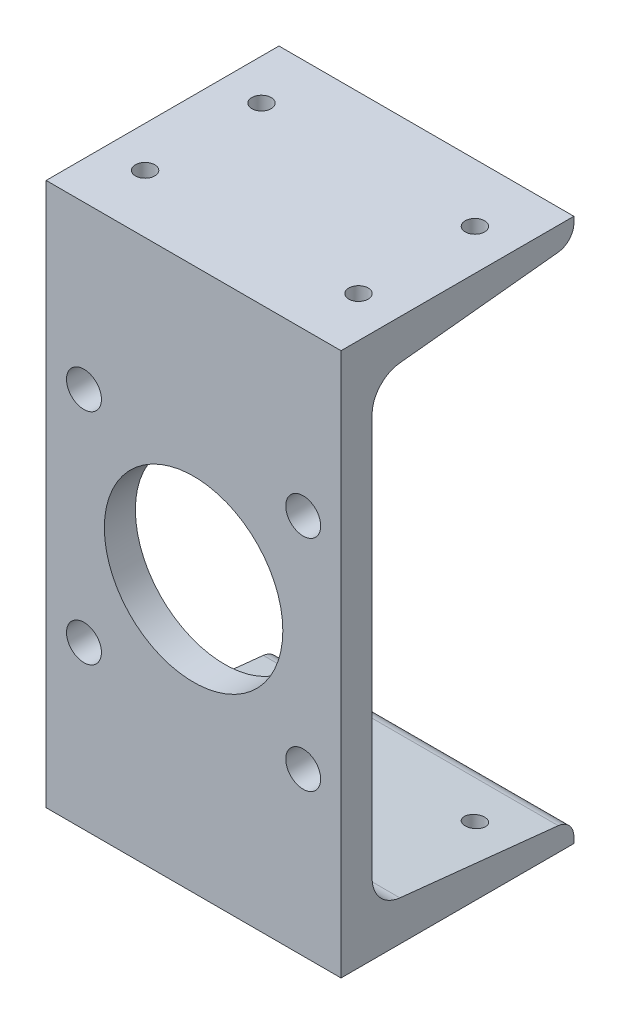
SolidWorks part; units mm, degrees
ref_plane "前视" through (0, 0, 0) normal (0, 0, 1) x (1, 0, 0)
ref_plane "上视" through (0, 0, 0) normal (0, 1, 0) x (1, 0, 0)
ref_plane "右视" through (0, 0, 0) normal (1, 0, 0) x (0, 0, -1)
sketch3d "3D草图1"
  line L0 (0, 0, 0) -> (76, 0, 0)
  dimension "D1" = 76
other "结构构件1"
ref_plane "基准面2" through (0, 0, 0) normal (1, 0, 0) x (0, 0, -1)
sketch "Sketch11" plane through (0, 0, 0) normal (1, 0, 0) x (0, 0, -1)
  line L0 (60, 140) -> (0, 140)
  line L1 (60, 0) -> (0, 0)
  line L2 (0, 140) -> (0, 0)
  line L6 (60, 140) -> (60, 138.4605)
  line L7 (60, 0) -> (60, 1.5395)
  line L12 (8, 121.74) -> (8, 18.26)
  line L17 (15.1638, 129.6962) -> (55.9704, 133.9851)
  line L18 (15.1638, 10.3038) -> (55.9704, 6.0149)
  arc A0 (55.9704, 133.9851) -> (60, 138.4605) centre (55.5, 138.4605) ccw
  arc A1 (55.9704, 6.0149) -> (60, 1.5395) centre (55.5, 1.5395) cw
  arc A9 (8, 18.26) -> (15.1638, 10.3038) centre (16, 18.26) ccw
  arc A10 (8, 121.74) -> (15.1638, 129.6962) centre (16, 121.74) cw
  point P8 (0, 70)
  point P9 (8, 70)
  point P10 (30, 140)
  point P11 (30, 0)
  point P12 (60, 5.5913)
  point P13 (60, 134.4087)
  point P14 (0, 0)
  dimension "D4" = 4.5
  dimension "RI" = 8
  dimension "D2" = 6
  dimension "D1" = 18.26
  dimension "D3" = 18.26
  dimension "Depth" = 140
  dimension "BF" = 60
  dimension "TW" = 8
sketch "草图4" plane through (0, 0, 0) normal (0, 0, 1) x (1, 0, 0)
  line L0 (76, 70) -> (0, 70) construction
  line L1 (76, 140) -> (76, 0) construction
  line L2 (0, 140) -> (0, 0) construction
  circle A0 centre (38, 70) radius 23
  dimension "D1" = 46
extrude "切除-拉伸1" cut sketch "草图4" against normal through all
sketch "草图6" plane through (0, 0, 0) normal (0, 0, 1) x (1, 0, 0)
  line L1 (66.25, 98.25) -> (9.75, 98.25) construction
  line L2 (66.25, 98.25) -> (66.25, 41.75) construction
  line L3 (66.25, 41.75) -> (9.75, 41.75) construction
  line L4 (9.75, 98.25) -> (9.75, 41.75) construction
  line L5 (66.25, 98.25) -> (9.75, 41.75) construction
  line L6 (66.25, 41.75) -> (9.75, 98.25) construction
  circle A0 centre (66.25, 41.75) radius 4.5
  circle A1 centre (9.75, 41.75) radius 4.5
  circle A2 centre (66.25, 98.25) radius 4.5
  circle A3 centre (9.75, 98.25) radius 4.5
  point P0 (38, 70)
  dimension "D1" = 9
  dimension "D2" = 56.5
extrude "切除-拉伸2" cut sketch "草图6" against normal through all
hole_wizard "M6 螺纹孔1" positions "草图8" profile "草图7" tap size "M6" standard "GB" end condition through all
sketch "草图8" plane through (0, 0, 0) normal (0, -1, 0) x (-1, 0, 0)
  line L0 (-65.5, 15) -> (-65.5, 45) construction
  line L1 (-65.5, 45) -> (-10.5, 45) construction
  line L2 (-10.5, 45) -> (-10.5, 15) construction
  line L3 (-10.5, 15) -> (-65.5, 15) construction
  line L6 (-38, 45) -> (-38, 60) construction
  line L7 (-76, 60) -> (0, 60) construction
  line L8 (-76, 30) -> (-65.5, 30) construction
  line L9 (-76, 0) -> (-76, 60) construction
  point P0 (-65.5, 15)
  point P2 (-65.5, 45)
  point P4 (-10.5, 15)
  point P6 (-10.5, 45)
  dimension "D1" = 30
  dimension "D2" = 55
sketch "草图7" plane through (65.5, 0, -15) normal (1, 0, 0) x (0, 0, -1)
  line L0 (0, 0) -> (0, 140)
  line L1 (0, 140) -> (2.5, 140)
  line L2 (2.5, 140) -> (2.5, 0)
  line L5 (2.5, 0) -> (0, 0)
  line L11 (0, -6.35) -> (0, 107.95) construction
  dimension "通孔螺纹孔钻头直径" = 5
  dimension "通孔螺纹孔钻头深度" = 140
cosmetic thread "孔螺蚊线1" parameters "D2"=6
cosmetic thread "孔螺蚊线2" parameters "D2"=6
cosmetic thread "孔螺蚊线3" parameters "D2"=6
cosmetic thread "孔螺蚊线4" parameters "D2"=6
